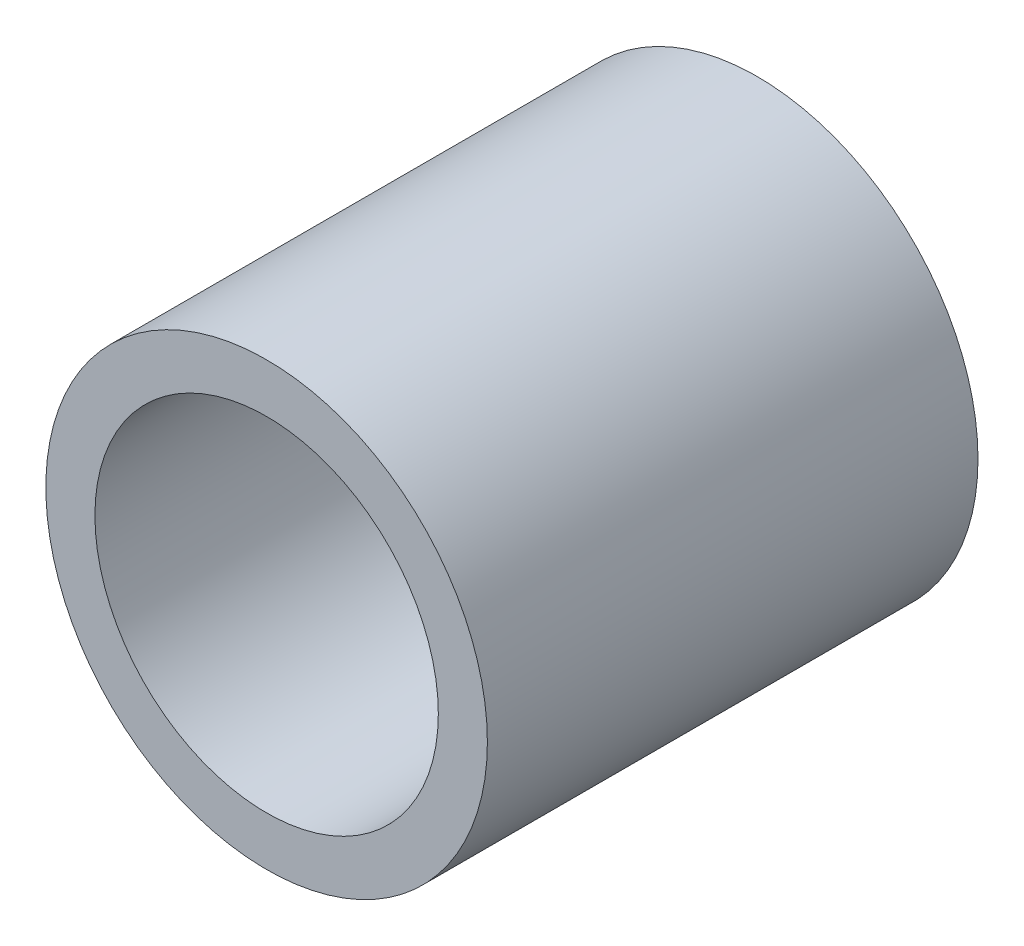
from build123d import *

# Parameters (mm, degrees)
SKETCH_1_R          = 20
SKETCH_1_R_2        = 15
EXTRUDE_1_DEPTH     = 50
EXTRUDE_START       = -50
SKETCH_2_R          = 22.5
SKETCH_2_R_2        = 20
EXTRUDE_2_DEPTH     = 50
SKETCH_3_R          = 17.5
CUT_EXTRUDE_2_DEPTH = 50


with BuildPart() as part:
    # 草图1 → 凸台-拉伸1 (new body)
    with BuildSketch(Plane.XY):
        Circle(SKETCH_1_R)
        Circle(SKETCH_1_R_2, mode=Mode.SUBTRACT)
    extrude(amount=EXTRUDE_1_DEPTH)

    # 草图2 → 凸台-拉伸2 (add)
    with BuildSketch(Plane.XY.offset(50).offset(EXTRUDE_START)):
        Circle(SKETCH_2_R)
        Circle(SKETCH_2_R_2, mode=Mode.SUBTRACT)
    extrude(amount=EXTRUDE_2_DEPTH)

    # 草图3 → 切除-拉伸2 (cut)
    with BuildSketch(Plane.XY.offset(50)):
        Circle(SKETCH_3_R)
    extrude(amount=-CUT_EXTRUDE_2_DEPTH, mode=Mode.SUBTRACT)


solid = part.part
